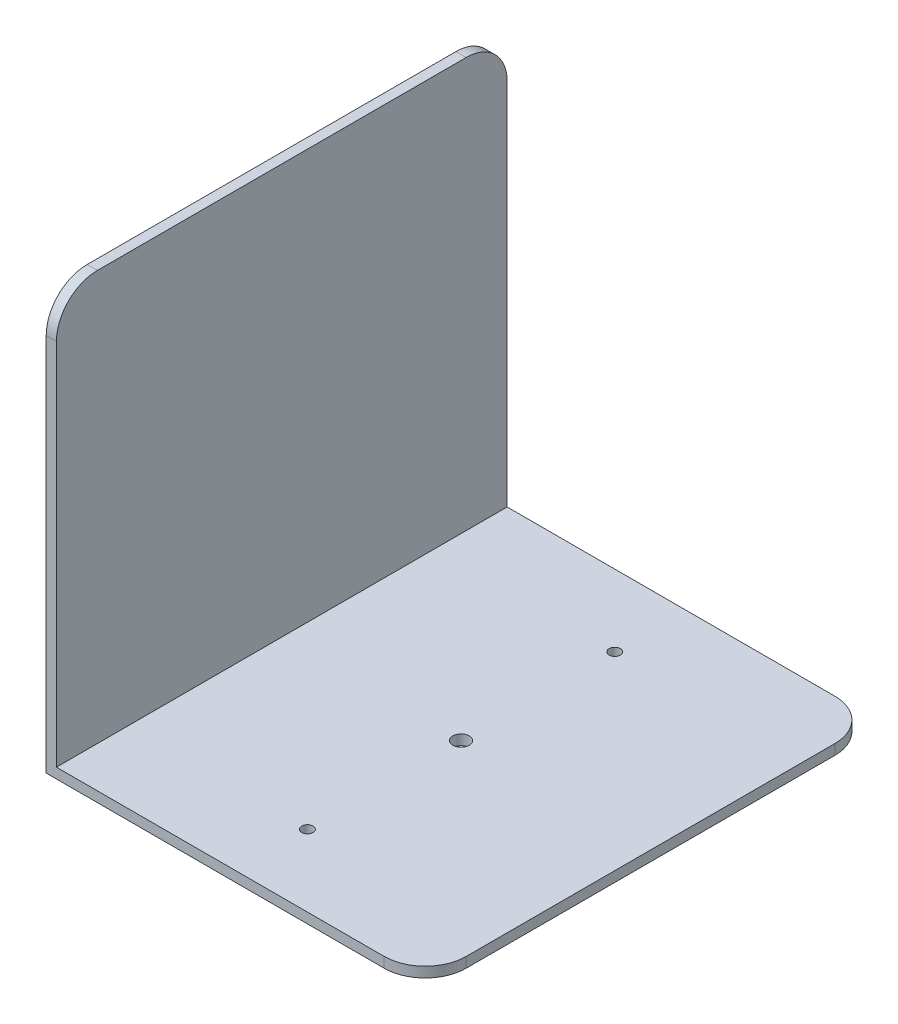
from build123d import *

# Parameters (mm, degrees)
SKETCH_1_W          = 370
SKETCH_1_H          = 440
EXTRUDE_1_DEPTH     = 5
CUT_EXTRUDE_1_REACH = 289.62
SKETCH_2_R          = 8
SKETCH_2_R_2        = 5.5
SKETCH_3_W          = 10
SKETCH_3_H          = 440
EXTRUDE_2_DEPTH     = 400
FILLET_1_R          = 40


with BuildPart() as part:
    # 草图1 → 凸台-拉伸1 (new, symmetric)
    with BuildSketch(Plane(origin=(0, 0, 0), x_dir=(1, 0, 0), z_dir=(0, 1, 0))):
        Rectangle(SKETCH_1_W, SKETCH_1_H)
    extrude(amount=EXTRUDE_1_DEPTH, both=True)

    # 草图2 → 切除-拉伸1 (cut, up to next)
    with BuildSketch(Plane(origin=(0, 5, 0), x_dir=(1, 0, 0), z_dir=(0, 1, 0)), mode=Mode.PRIVATE) as cut_extrude_1_sk1:
        with Locations(Location((0, 0, 0), (0, 0, 270))):
            Circle(SKETCH_2_R)
    cut_extrude_1_tool1 = extrude(cut_extrude_1_sk1.sketch, amount=-CUT_EXTRUDE_1_REACH, mode=Mode.PRIVATE) & part.part
    # 草图2 → 切除-拉伸1 (cut, up to next)
    with BuildSketch(Plane(origin=(0, 5, 0), x_dir=(1, 0, 0), z_dir=(0, 1, 0)), mode=Mode.PRIVATE) as cut_extrude_1_sk2:
        with Locations(Location((0, 150, 0), (0, 0, 270))):
            Circle(SKETCH_2_R_2)
    cut_extrude_1_tool2 = extrude(cut_extrude_1_sk2.sketch, amount=-CUT_EXTRUDE_1_REACH, mode=Mode.PRIVATE) & part.part
    # 草图2 → 切除-拉伸1 (cut, up to next)
    with BuildSketch(Plane(origin=(0, 5, 0), x_dir=(1, 0, 0), z_dir=(0, 1, 0)), mode=Mode.PRIVATE) as cut_extrude_1_sk3:
        with Locations(Location((0, -150, 0), (0, 0, 270))):
            Circle(SKETCH_2_R_2)
    cut_extrude_1_tool3 = extrude(cut_extrude_1_sk3.sketch, amount=-CUT_EXTRUDE_1_REACH, mode=Mode.PRIVATE) & part.part
    add(cut_extrude_1_tool1.solids().sort_by_distance((0, 5, 0))[0], mode=Mode.SUBTRACT)
    add(cut_extrude_1_tool2.solids().sort_by_distance((0, 5, -150))[0], mode=Mode.SUBTRACT)
    add(cut_extrude_1_tool3.solids().sort_by_distance((0, 5, 150))[0], mode=Mode.SUBTRACT)

    # 草图3 → 凸台-拉伸2 (add)
    with BuildSketch(Plane(origin=(0, 5, 0), x_dir=(1, 0, 0), z_dir=(0, 1, 0))):
        with Locations((-180, 0)):
            Rectangle(SKETCH_3_W, SKETCH_3_H)
    extrude(amount=EXTRUDE_2_DEPTH)

    # 圆角1
    fillet_1_edges = [part.edges().sort_by_distance(p)[0] for p in [
        (-180, 405, 220),
        (-180, 405, -220),
        (185, 0, 220),
        (185, 0, -220),
    ]]
    fillet(fillet_1_edges, radius=FILLET_1_R)


solid = part.part
